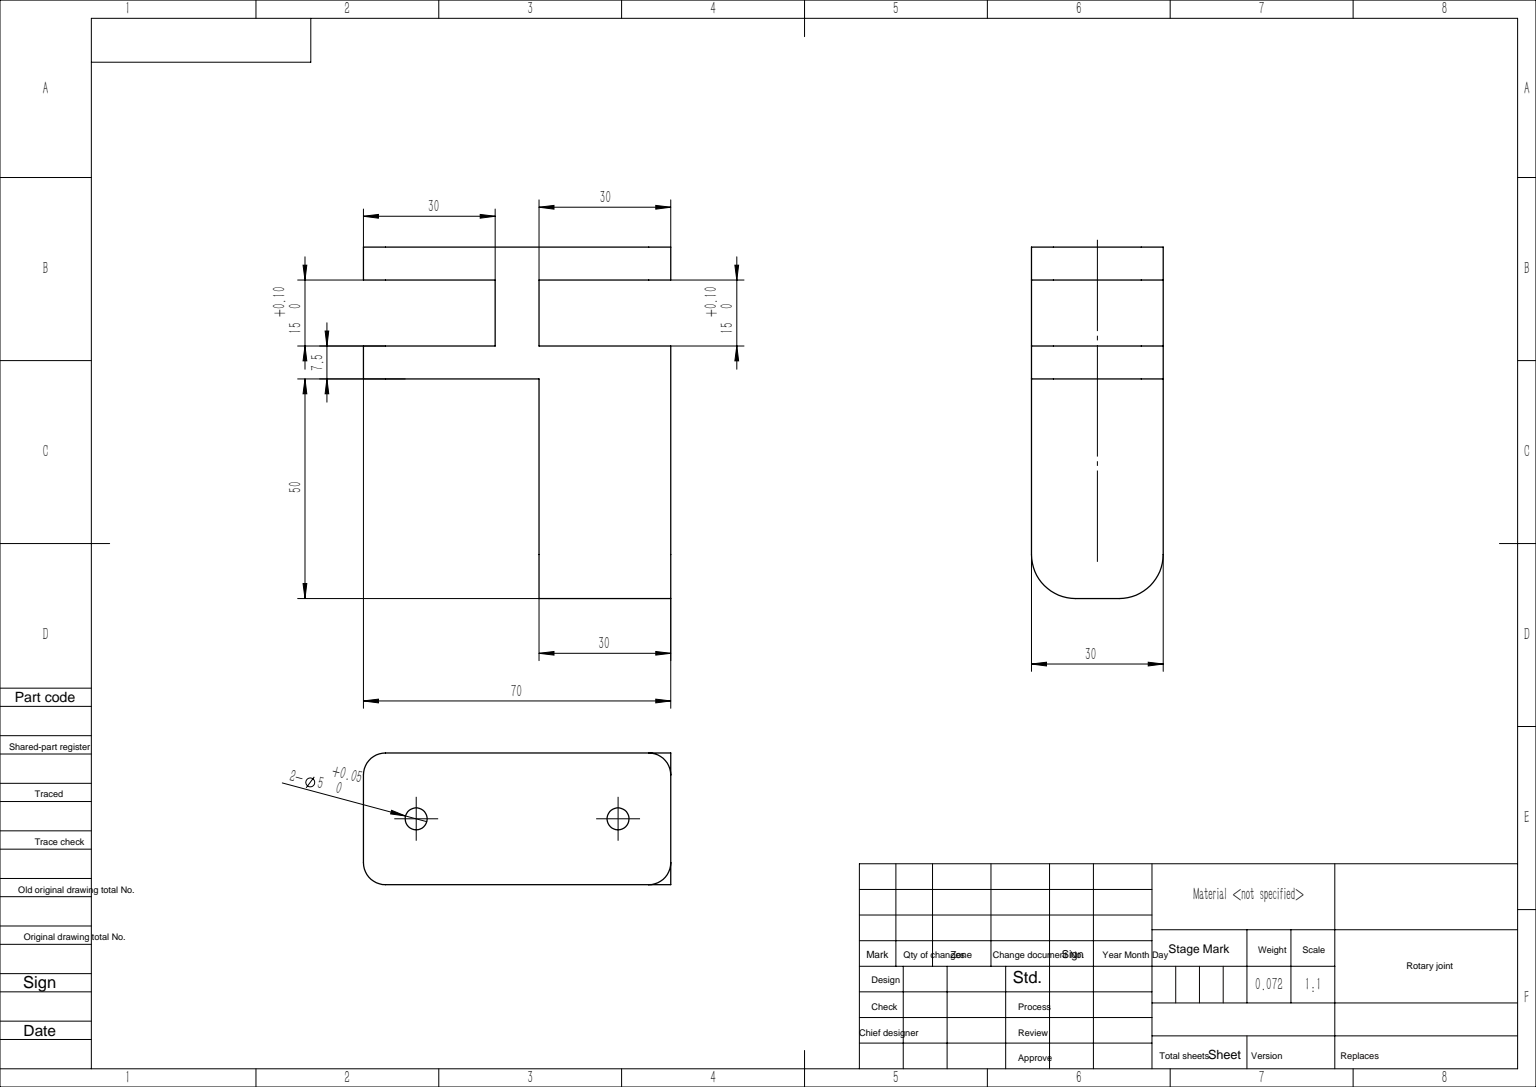
from build123d import *

# Parameters (mm, degrees)
BOSS_EXTRUDE1_DEPTH = 30
SKETCH4_R           = 9
CUT_EXTRUDE2_DEPTH  = 25
SKETCH5_W           = 15
SKETCH5_H           = 30
CUT_EXTRUDE3_DEPTH  = 111.453610172
SKETCH6_R           = 2.5
CUT_EXTRUDE4_DEPTH  = 25
FILLET1_R           = 5
FILLET2_R           = 10


with BuildPart() as part:
    # Sketch1 → Boss-Extrude1 (new body)
    with BuildSketch(Plane.XY):
        Polygon((0, 0), (0, 70), (30, 70), (30, 30), (80, 30), (80, 0), align=None)
    extrude(amount=BOSS_EXTRUDE1_DEPTH)

    # Sketch4 → Cut-Extrude2 (cut)
    with BuildSketch(Plane(origin=(0, 0, 0), x_dir=(-1, 0, 0), z_dir=(0, -1, 0))):
        with Locations(Location((-65, -15, 0), (0, 0, 180))):
            Circle(SKETCH4_R)
    extrude(amount=-CUT_EXTRUDE2_DEPTH, mode=Mode.SUBTRACT)

    # Sketch5 → Cut-Extrude3 (cut, through all)
    with BuildSketch(Plane(origin=(0, 0, 0), x_dir=(-1, 0, 0), z_dir=(0, 0, -1))):
        with Locations((-15, 55)):
            Rectangle(SKETCH5_W, SKETCH5_H)
        with Locations((-15, 15)):
            Rectangle(SKETCH5_W, SKETCH5_H)
    extrude(amount=-CUT_EXTRUDE3_DEPTH, mode=Mode.SUBTRACT)

    # Sketch6 → Cut-Extrude4 (cut, symmetric)
    with BuildSketch(Plane.ZY.offset(-22.5)):
        with Locations(Location((15, 58, 0), (0, 0, 270))):
            Circle(SKETCH6_R)
        with Locations((15, 12)):
            Circle(SKETCH6_R)
    extrude(amount=CUT_EXTRUDE4_DEPTH, both=True, mode=Mode.SUBTRACT)

    # Fillet1
    fillet1_edges = [part.edges().sort_by_distance(p)[0] for p in [
        (26.25, 70, 30),
        (3.75, 70, 0),
        (3.75, 70, 30),
        (3.75, 0, 30),
        (26.25, 70, 0),
        (3.75, 0, 0),
    ]]
    fillet(fillet1_edges, radius=FILLET1_R)

    # Fillet2
    fillet2_edges = [part.edges().sort_by_distance(p)[0] for p in [
        (80, 15, 30),
        (80, 15, 0),
    ]]
    fillet(fillet2_edges, radius=FILLET2_R)


solid = part.part
